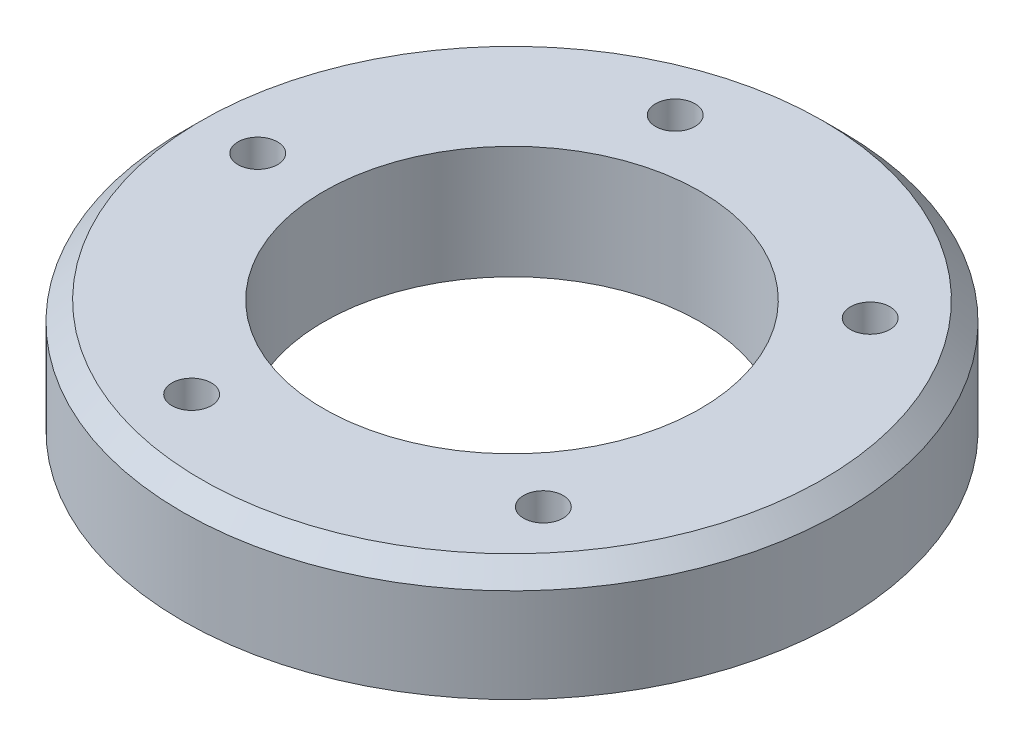
SolidWorks part; units mm, degrees
material "Q235B"
ref_plane "Front Plane" through (0, 0, 0) normal (0, 0, 1) x (1, 0, 0)
ref_plane "Top Plane" through (0, 0, 0) normal (0, 1, 0) x (1, 0, 0)
ref_plane "Right Plane" through (0, 0, 0) normal (1, 0, 0) x (0, 0, -1)
sketch "Sketch1" plane through (0, 0, 0) normal (1, 0, 0) x (0, 0, -1)
  line L0 (0, 0) -> (0, 27.6874) construction
  line L1 (35, 10) -> (33, 12)
  line L2 (20, 0) -> (35, 0)
  line L3 (35, 0) -> (35, 10)
  line L6 (33, 12) -> (20, 12)
  line L7 (20, 12) -> (20, 0)
  point P6 (35, 12)
  dimension "D1" = 40
  dimension "D2" = 12
  dimension "D3" = 70
revolve "Revolve1" add sketch "Sketch1" angle 360 about L0
sketch "Sketch2" plane through (0, 12, 0) normal (0, 1, 0) x (1, 0, 0)
  line L0 (0, 0) -> (-27, 0) construction
  line L1 (0, 0) -> (0, 27) construction
  line L2 (0, 0) -> (-8.3435, 25.6785) construction
  line L3 (0, 0) -> (20.6832, 17.3553) construction
  line L4 (0, 0) -> (-8.3435, -25.6785) construction
  line L5 (0, 0) -> (20.6832, -17.3553) construction
  circle A0 centre (-27, 0) radius 1.75
  circle A1 centre (0, 0) radius 27 construction
  circle A2 centre (-8.3435, 25.6785) radius 1.75
  circle A3 centre (-8.3435, -25.6785) radius 1.75
  circle A4 centre (20.6832, 17.3553) radius 1.75
  circle A5 centre (20.6832, -17.3553) radius 1.75
  dimension "D1" = 54
  dimension "D2" = 3.5
  dimension "D3" = 72
  dimension "D4" = 68
  dimension "D5" = 72
extrude "Cut-Extrude1" cut sketch "Sketch2" against normal blind 10
hole_wizard "M5 Tapped Hole1" positions "Sketch3" profile "Sketch4" tap size "M5" standard "GB"
sketch "Sketch3" plane through (0, 12, 0) normal (0, 1, 0) x (1, 0, 0)
  point P0 (-27, 0)
  point P3 (-8.3435, 25.6785)
  point P6 (20.6832, 17.3553)
  point P9 (20.6832, -17.3553)
  point P12 (-8.3435, -25.6785)
sketch "Sketch4" plane through (-27, 12, 0) normal (1, 0, 0) x (0, 0, 1)
  line L0 (0, 0) -> (0, 11.2618)
  line L1 (0, 11.2618) -> (2.1, 10)
  line L2 (2.1, 10) -> (2.1, 0)
  line L5 (2.1, 0) -> (0, 0)
  line L10 (0, 11.2618) -> (-2.1, 10) construction
  line L11 (0, -6.35) -> (0, 107.95) construction
  dimension "螺纹孔钻头直径" = 4.2
  dimension "螺纹孔钻头深度" = 10
  dimension "导头角度" = 118
cosmetic thread "Hole Cosmetic Thread1" parameters "D1"=6, "D2"=5
cosmetic thread "Hole Cosmetic Thread2" parameters "D1"=6, "D2"=5
cosmetic thread "Hole Cosmetic Thread3" parameters "D1"=6, "D2"=5
cosmetic thread "Hole Cosmetic Thread4" parameters "D1"=6, "D2"=5
cosmetic thread "Hole Cosmetic Thread5" parameters "D1"=6, "D2"=5
